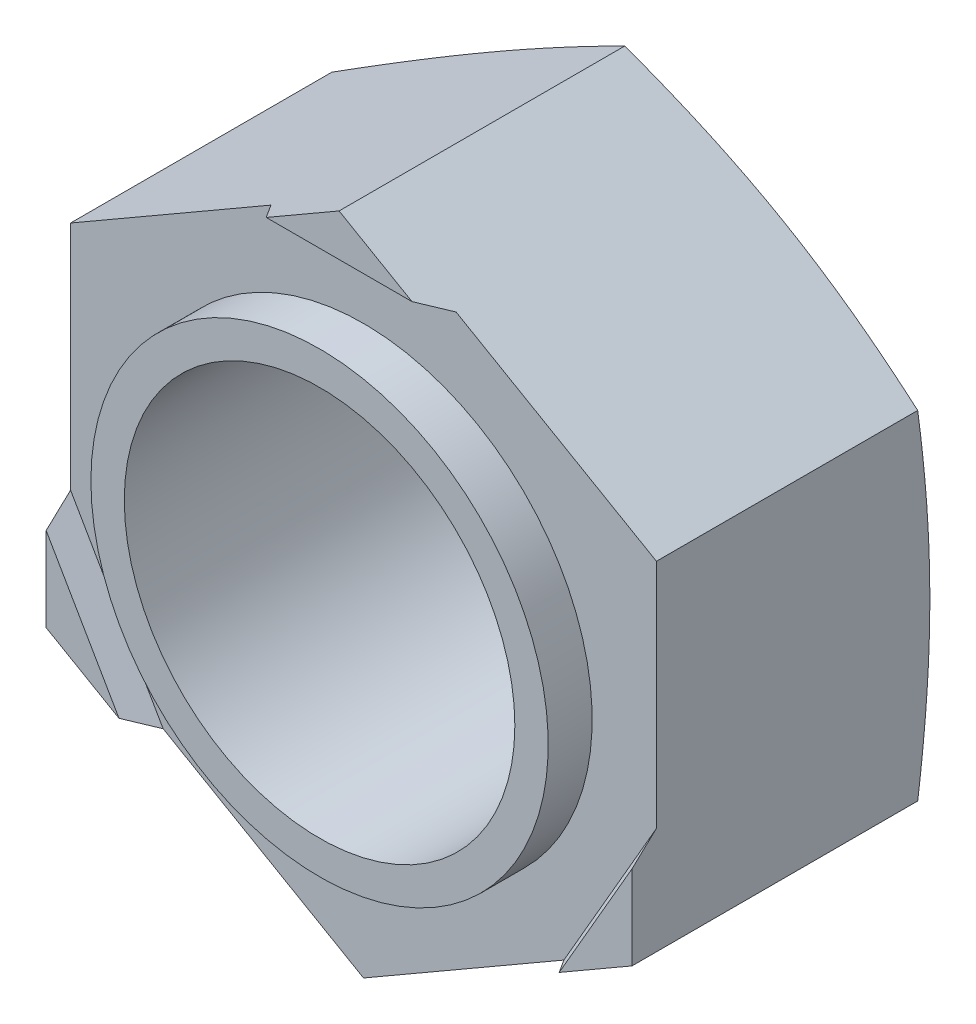
from build123d import *

# Parameters (mm, degrees)
SKETCH_1_R               = 8
EXTRUDE_1_DEPTH          = 13
CUT_EXTRUDE_2_DEPTH      = 23.472205054
PATTERN_CIRCULAR_1_COUNT = 3
SKETCH_2_R               = 9.3675
SKETCH_2_R_2             = 8
EXTRUDE_2_DEPTH          = 1.8
SKETCH_4_OUTSIDE_W       = 208.978
SKETCH_4_OUTSIDE_H       = 212.69
SKETCH_4_OUTSIDE_R       = 12
CUT_EXTRUDE_3_DEPTH      = 23.472205054
CUT_EXTRUDE_3_DRAFT      = -75
SKETCH_5_R               = 9.565
CUT_EXTRUDE_4_DEPTH      = 0.2


with BuildPart() as part:
    # 草图1 → 拉伸1 (new body)
    with BuildSketch(Plane.XY):
        Polygon((0, 13.856406461), (-12, 6.92820323), (-12, -6.92820323), (0, -13.856406461), (12, -6.92820323), (12, 6.92820323), align=None)
        with Locations(Location((0, 0, 0), (0, 0, 180))):
            Circle(SKETCH_1_R, mode=Mode.SUBTRACT)
    extrude(amount=EXTRUDE_1_DEPTH)

    # 草图3 → 切除-拉伸2 (cut, symmetric)
    with BuildSketch(Plane(origin=(0, 0, 0), x_dir=(0, 0, -1), z_dir=(1, 0, 0))):
        Polygon((-12.2, 12.133037667), (-11.2, 11.666730008), (-11.2, 0), (-13, 0), (-13, 13.856406461), (-12.2, 13.856406461), align=None)
    cut_extrude_2 = extrude(amount=CUT_EXTRUDE_2_DEPTH, both=True, mode=Mode.SUBTRACT)

    # 阵列(圆周)1: 切除-拉伸2 ×3 about axis
    pattern_circular_1_axis = Axis((0, 0, 0), (0, 0, 1))
    for i in range(1, PATTERN_CIRCULAR_1_COUNT):
        add(cut_extrude_2.rotate(pattern_circular_1_axis, i * 360 / PATTERN_CIRCULAR_1_COUNT), mode=Mode.SUBTRACT)

    # 草图2 → 拉伸2 (add)
    with BuildSketch(Plane.XY.offset(11.2)):
        with Locations(Location((0, 0, 0), (0, 0, 180))):
            Circle(SKETCH_2_R)
        with Locations(Location((0, 0, 0), (0, 0, 180))):
            Circle(SKETCH_2_R_2, mode=Mode.SUBTRACT)
    extrude(amount=EXTRUDE_2_DEPTH)


with BuildPart() as cut_extrude_3_tool:
    # 草图4 outside → 切除-拉伸3 (with draft: the straight prism first)
    with BuildSketch(Plane(origin=(0, 0, 0), x_dir=(-1, 0, 0), z_dir=(0, 0, -1))):
        Rectangle(SKETCH_4_OUTSIDE_W, SKETCH_4_OUTSIDE_H)
        Circle(SKETCH_4_OUTSIDE_R, mode=Mode.SUBTRACT)
    extrude(amount=-CUT_EXTRUDE_3_DEPTH)
    # 切除-拉伸3: the draft: its side faces are tilted about the plane it starts from
    cut_extrude_3_sides = [cut_extrude_3_tool.faces().sort_by_distance(p)[0] for p in [
        (0, -106.345, 11.736102527),
        (-104.489, 0, 11.736102527),
        (0, 106.345, 11.736102527),
        (104.489, 0, 11.736102527),
        (12, 0, 11.736102527),
    ]]
    draft(cut_extrude_3_sides, Plane(origin=(0, 0, 0), x_dir=(-1, 0, 0), z_dir=(0, 0, -1)), CUT_EXTRUDE_3_DRAFT)


with BuildPart() as part_1:
    add(part.part)

    # 切除-拉伸3: cut by cut_extrude_3_tool
    add(cut_extrude_3_tool.part, mode=Mode.SUBTRACT)

    # 草图5 → 切除-拉伸4 (cut)
    with BuildSketch(Plane(origin=(0, 0, 0), x_dir=(-1, 0, 0), z_dir=(0, 0, -1))):
        Circle(SKETCH_5_R)
    extrude(amount=-CUT_EXTRUDE_4_DEPTH, mode=Mode.SUBTRACT)


solid = part_1.part
